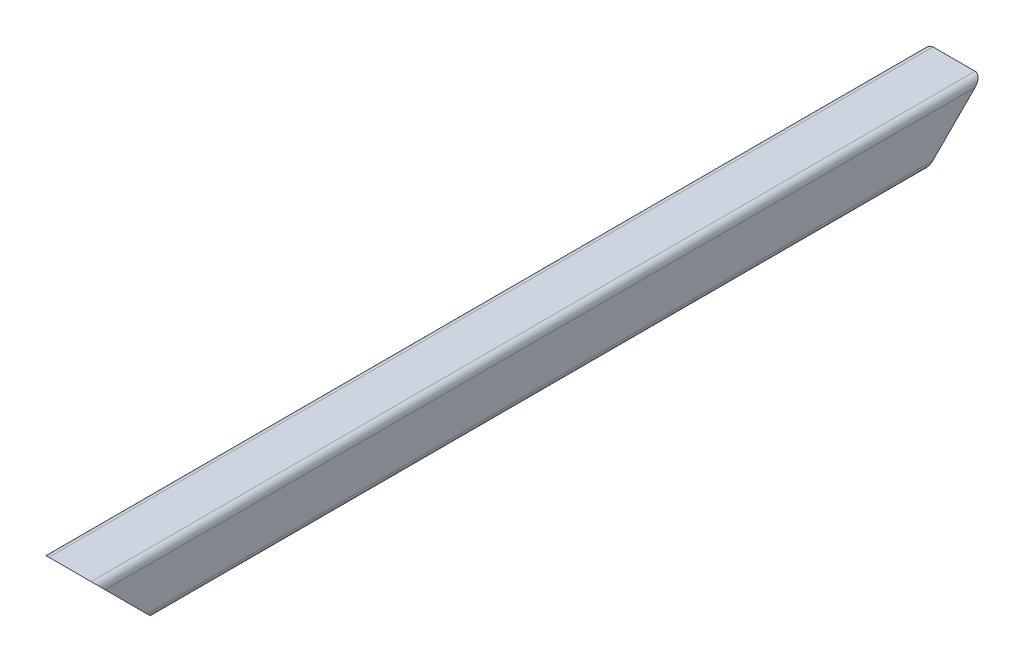
from build123d import *

# Parameters (mm, degrees)
BOSS_EXTRUDE_1_DEPTH     = 503.38
CUT_EXTRUDE_1_DEPTH      = 506.410154627
CUT_EXTRUDE_1_DEPTH_BACK = 506.410154627


with BuildPart() as part:
    # Sketch 1 → Boss-Extrude 1 (new, symmetric)
    with BuildSketch(Plane.XY):
        with BuildLine():
            Line((0, 32), (-24, 32))
            ThreePointArc((-24, 32), (-29.656854249, 29.656854249), (-32, 24))
            Line((-32, 24), (-32, 0))
            Line((-32, 0), (-32, -24))
            ThreePointArc((-32, -24), (-29.656854249, -29.656854249), (-24, -32))
            Line((-24, -32), (24, -32))
            ThreePointArc((24, -32), (29.656854249, -29.656854249), (32, -24))
            Line((32, -24), (32, 0))
            Line((32, 0), (32, 24))
            ThreePointArc((32, 24), (29.656854249, 29.656854249), (24, 32))
            Line((24, 32), (0, 32))
        make_face()
        with BuildLine():
            Line((0, 28), (-24, 28))
            ThreePointArc((-24, 28), (-26.828427125, 26.828427125), (-28, 24))
            Line((-28, 24), (-28, 0))
            Line((-28, 0), (-28, -24))
            ThreePointArc((-28, -24), (-26.828427125, -26.828427125), (-24, -28))
            Line((-24, -28), (24, -28))
            ThreePointArc((24, -28), (26.828427125, -26.828427125), (28, -24))
            Line((28, -24), (28, 0))
            Line((28, 0), (28, 24))
            ThreePointArc((28, 24), (26.828427125, 26.828427125), (24, 28))
            Line((24, 28), (0, 28))
        make_face(mode=Mode.SUBTRACT)
    extrude(amount=BOSS_EXTRUDE_1_DEPTH, both=True)

    # Sketch 2 → Cut-Extrude 1 (cut, two sides: drawn at the far end of the back side and taken through both)
    with BuildSketch(Plane(origin=(0, 0, 0), x_dir=(0, 0, -1), z_dir=(1, 0, 0)).offset(-CUT_EXTRUDE_1_DEPTH_BACK)):
        Polygon((-503.38, 32), (-439.38, -32), (-503.38, -32), align=None)
        Polygon((503.38, -32), (503.38, 32), (439.38, -32), align=None)
    extrude(amount=CUT_EXTRUDE_1_DEPTH + CUT_EXTRUDE_1_DEPTH_BACK, mode=Mode.SUBTRACT)


solid = part.part
